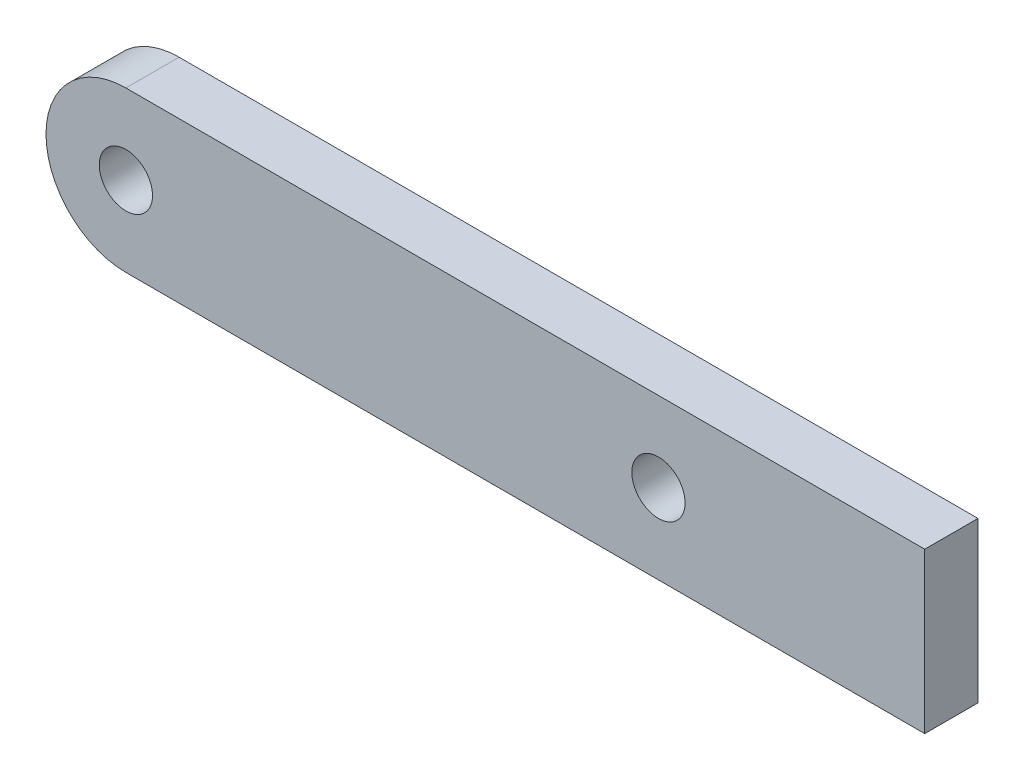
from build123d import *

# Parameters (mm, degrees)
SKETCH1_R           = 50
BOSS_EXTRUDE1_DEPTH = 100


with BuildPart() as part:
    # Sketch1 → Boss-Extrude1 (new body)
    with BuildSketch(Plane.XY):
        with BuildLine():
            Line((0, 150), (1500, 150))
            Line((1500, 150), (1500, -150))
            Line((1500, -150), (0, -150))
            ThreePointArc((0, -150), (-150, 0), (0, 150))
        make_face()
        with Locations((1000, 0)):
            Circle(SKETCH1_R, mode=Mode.SUBTRACT)
        Circle(SKETCH1_R, mode=Mode.SUBTRACT)
    extrude(amount=BOSS_EXTRUDE1_DEPTH)


solid = part.part
